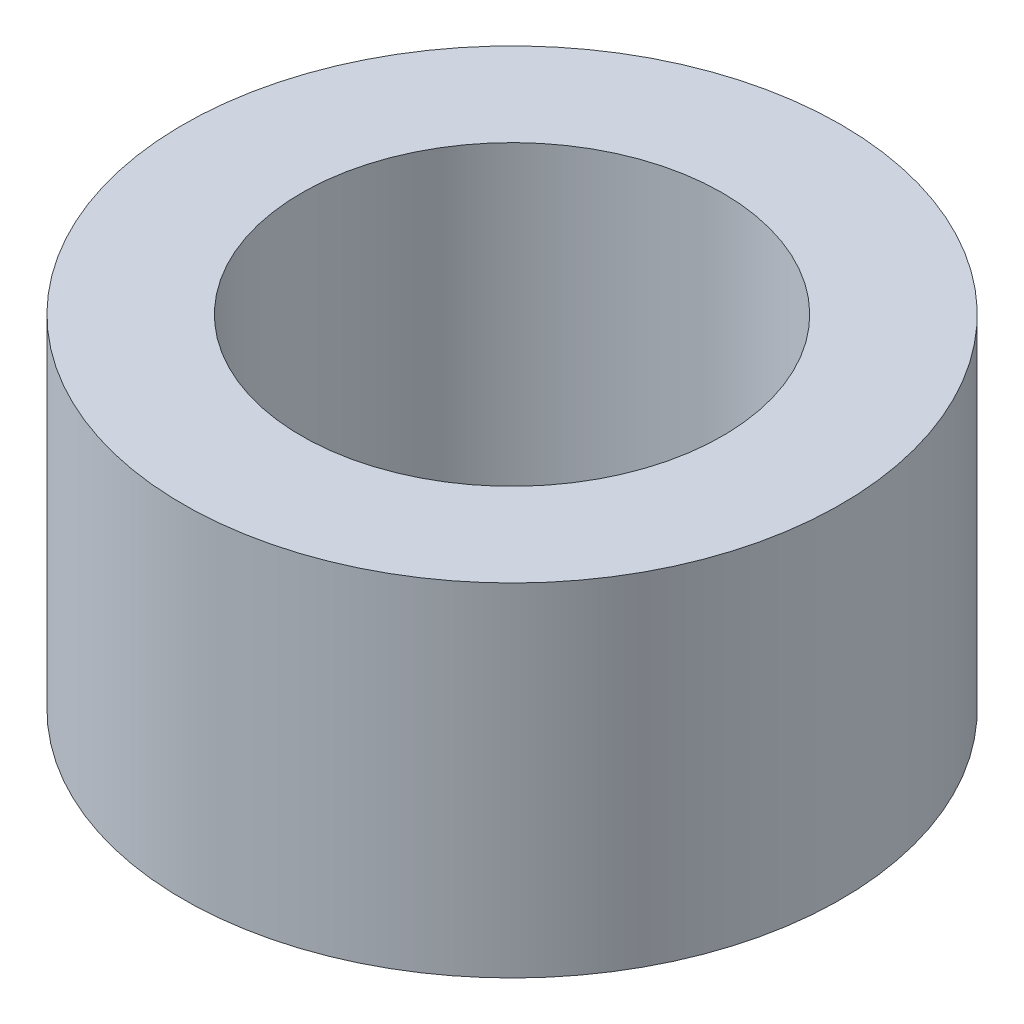
from build123d import *

# Parameters (mm, degrees)
SKETCH_1_R      = 12.5
SKETCH_1_R_2    = 8
EXTRUDE_1_DEPTH = 13


with BuildPart() as part:
    # 草图1 → 凸台-拉伸1 (new body)
    with BuildSketch(Plane(origin=(0, 0, 0), x_dir=(1, 0, 0), z_dir=(0, 1, 0))):
        with Locations(Location((0, 0, 0), (0, 0, 90))):
            Circle(SKETCH_1_R)
        with Locations(Location((0, 0, 0), (0, 0, 90))):
            Circle(SKETCH_1_R_2, mode=Mode.SUBTRACT)
    extrude(amount=EXTRUDE_1_DEPTH)


solid = part.part
